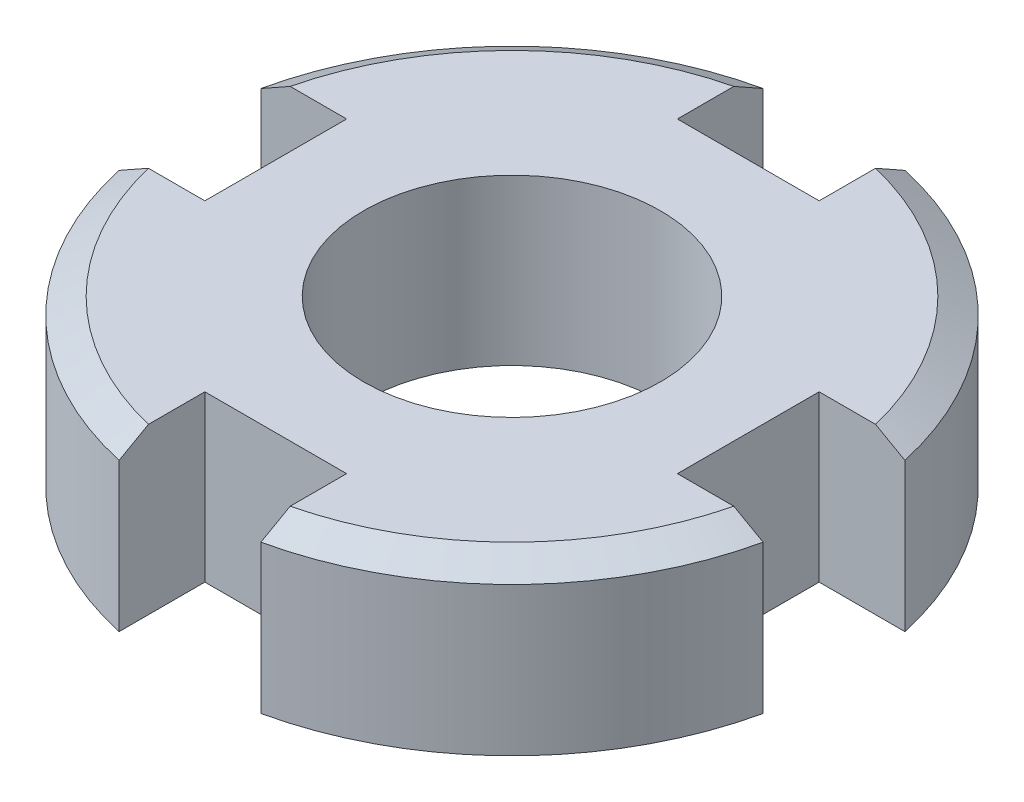
SolidWorks part; units mm, degrees
material "AISI 304"
ref_plane "前视基准面" through (0, 0, 0) normal (0, 0, 1) x (1, 0, 0)
ref_plane "上视基准面" through (0, 0, 0) normal (0, 1, 0) x (1, 0, 0)
ref_plane "右视基准面" through (0, 0, 0) normal (1, 0, 0) x (0, 0, -1)
sketch "草图1" plane through (0, 0, 0) normal (0, 1, 0) x (1, 0, 0)
  line L0 (0, 7.1661) -> (0, 0) construction
  line L1 (-2.15, 9.7661) -> (-2.15, 7.1661)
  line L2 (-2.15, 7.1661) -> (2.15, 7.1661)
  line L3 (2.15, 7.1661) -> (2.15, 9.7661)
  line L4 (9.7661, 2.15) -> (7.1661, 2.15)
  line L5 (7.1661, 2.15) -> (7.1661, -2.15)
  line L6 (7.1661, -2.15) -> (9.7661, -2.15)
  line L7 (2.15, -9.7661) -> (2.15, -7.1661)
  line L8 (2.15, -7.1661) -> (-2.15, -7.1661)
  line L9 (-2.15, -7.1661) -> (-2.15, -9.7661)
  line L10 (-9.7661, -2.15) -> (-7.1661, -2.15)
  line L11 (-7.1661, -2.15) -> (-7.1661, 2.15)
  line L12 (-7.1661, 2.15) -> (-9.7661, 2.15)
  arc A0 (-2.15, 9.7661) -> (-9.7661, 2.15) centre (0, 0) ccw
  arc A1 (-9.7661, -2.15) -> (-2.15, -9.7661) centre (0, 0) ccw
  arc A2 (2.15, -9.7661) -> (9.7661, -2.15) centre (0, 0) ccw
  arc A3 (9.7661, 2.15) -> (2.15, 9.7661) centre (0, 0) ccw
  point P22 (0, 0)
  dimension "D1" = 20
  dimension "D2" = 2.6
  dimension "D3" = 4.3
  dimension "D4" = 4
extrude "凸台-拉伸1" add sketch "草图1" along normal blind 5
sketch "草图2" plane through (0, 5, 0) normal (0, 1, 0) x (1, 0, 0)
  point P0 (0, 0)
hole_wizard "M10x1.0 螺纹孔1" positions "草图2" profile "草图3" tap size "M10x1.0" standard "GB" end condition through all
sketch "草图3" plane through (0, 5, 0) normal (1, 0, 0) x (0, 0, 1)
  line L0 (0, 0) -> (0, 5)
  line L1 (0, 5) -> (4.5, 5)
  line L2 (4.5, 5) -> (4.5, 0)
  line L5 (4.5, 0) -> (0, 0)
  line L11 (0, -6.35) -> (0, 107.95) construction
  dimension "通孔螺纹孔钻头直径" = 9
  dimension "通孔螺纹孔钻头深度" = 5
cosmetic thread "孔螺纹线1" parameters "D2"=10
chamfer "倒角1" distance 0.5 angle 60 4 edges at (-7.0711, 5, -7.0711) (7.0711, 5, -7.0711) (7.0711, 5, 7.0711) (-7.0711, 5, 7.0711)
